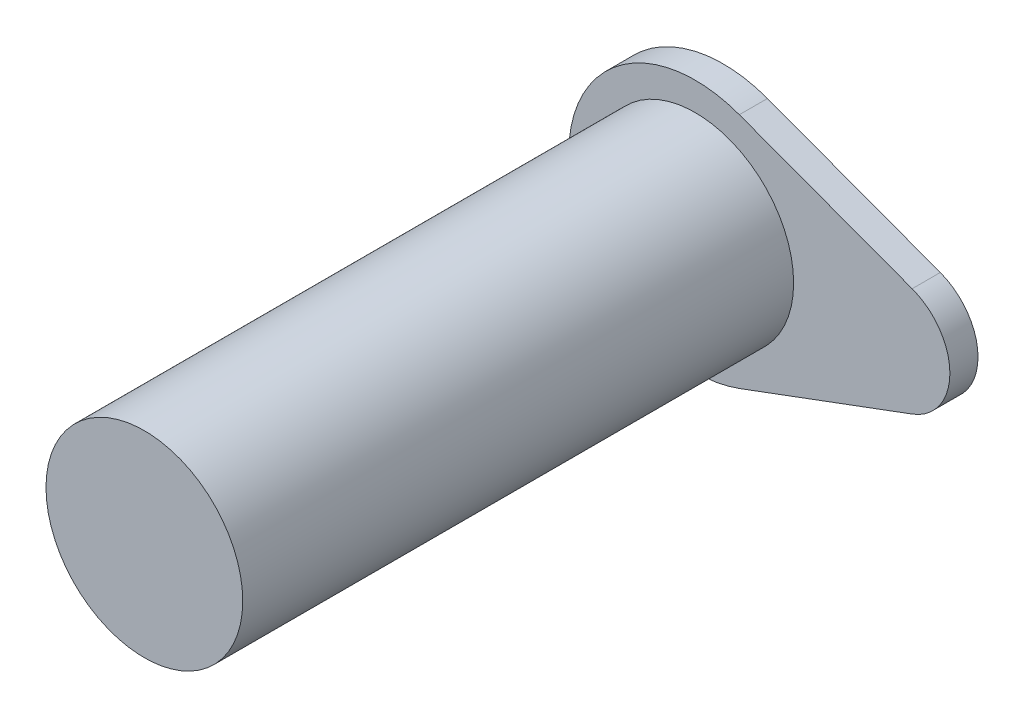
from build123d import *

# Parameters (mm, degrees)
SKETCH_1_R          = 17.5
EXTRUDE_1_DEPTH     = 103
SKETCH_2_R          = 17.5
EXTRUDE_3_DEPTH     = 5
SKETCH_3_R          = 4
CUT_EXTRUDE_1_DEPTH = 70
CUT_EXTRUDE_2_DEPTH = 70


with BuildPart() as part:
    # 草图1 → 凸台-拉伸1 (new body)
    with BuildSketch(Plane.XY):
        Circle(SKETCH_1_R)
    extrude(amount=EXTRUDE_1_DEPTH)

    # 草图2 → 凸台-拉伸3 (add)
    with BuildSketch(Plane(origin=(0, 0, 0), x_dir=(-1, 0, 0), z_dir=(0, 0, -1))):
        with BuildLine():
            Line((-7.842143419, 21.089115358), (-38.590345949, 9.655168982))
            ThreePointArc((-38.590345949, 9.655168982), (-45.301110237, 0), (-38.590345949, -9.655168982))
            Line((-38.590345949, -9.655168982), (-7.842143419, -21.089115358))
            ThreePointArc((-7.842143419, -21.089115358), (22.5, 0), (-7.842143419, 21.089115358))
        make_face()
        Circle(SKETCH_2_R, mode=Mode.SUBTRACT)
    extrude(amount=-EXTRUDE_3_DEPTH)

    # 草图3 → 切除-拉伸1 (cut)
    with BuildSketch(Plane(origin=(0, 0, 0), x_dir=(-1, 0, 0), z_dir=(0, 0, -1))):
        Circle(SKETCH_3_R)
    extrude(amount=-CUT_EXTRUDE_1_DEPTH, mode=Mode.SUBTRACT)

    # 草图4 → 切除-拉伸2 (cut)
    with BuildSketch(Plane(origin=(0, 0, 0), x_dir=(1, 0, 0), z_dir=(0, 1, 0))):
        with BuildLine():
            Line((0, -51.5), (0, -55.5))
            ThreePointArc((0, -55.5), (2.828427125, -54.328427125), (4, -51.5))
            Line((4, -51.5), (0, -51.5))
        make_face()
        with BuildLine():
            Line((0, -47.5), (0, -51.5))
            Line((0, -51.5), (4, -51.5))
            ThreePointArc((4, -51.5), (2.828427125, -48.671572875), (0, -47.5))
        make_face()
        with BuildLine():
            ThreePointArc((0, -47.5), (-4, -51.5), (0, -55.5))
            Line((0, -55.5), (0, -51.5))
            Line((0, -51.5), (0, -47.5))
        make_face()
    extrude(amount=-CUT_EXTRUDE_2_DEPTH, mode=Mode.SUBTRACT)


solid = part.part
